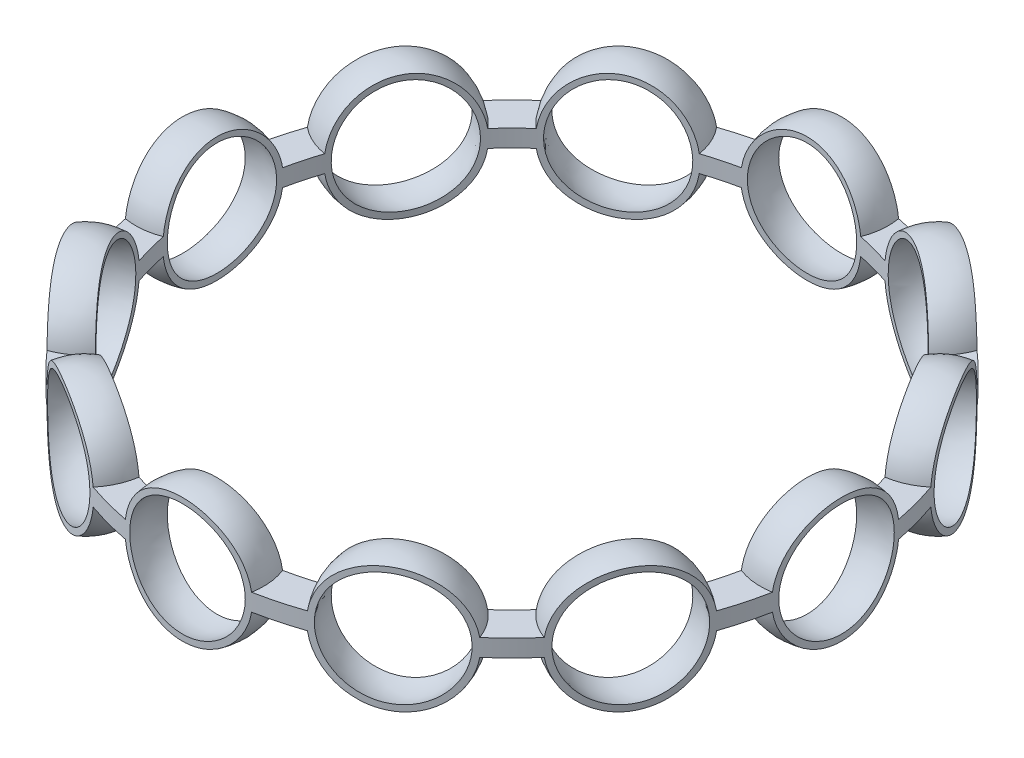
from build123d import *

# Parameters (mm, degrees)
SKETCH1_R               = 50
BOSS_EXTRUDE1_DEPTH     = 1
CIRPATTERN1_COUNT       = 12
CUT_EXTRUDE2_DEPTH      = 72.107313267
CUT_EXTRUDE2_DEPTH_BACK = 72.107313267
SKETCH3_OUTSIDE_W       = 130.442
SKETCH3_OUTSIDE_H       = 130.442
SKETCH3_OUTSIDE_R       = 38.25
SKETCH3_OUTSIDE_R_2     = 34.25
CIRPATTERN2_COUNT       = 12


with BuildPart() as part:
    # Sketch1 → Boss-Extrude1 (new, symmetric)
    with BuildSketch(Plane(origin=(0, 0, 0), x_dir=(1, 0, 0), z_dir=(0, 1, 0))):
        with Locations(Location((0, 0, 0), (0, 0, 270))):
            Circle(SKETCH1_R)
    extrude(amount=BOSS_EXTRUDE1_DEPTH, both=True)

    # Sketch2 → Revolve1 (revolve)
    with BuildSketch(Plane(origin=(0, 0, 0), x_dir=(0, 0, -1), z_dir=(1, 0, 0))):
        with BuildLine():
            Line((36.25, 7.5), (36.25, -7.5))
            ThreePointArc((36.25, -7.5), (43.75, 0), (36.25, 7.5))
        make_face()
    revolve1 = revolve(axis=Axis((0, 22.32089878, -36.25), (0, -1, 0)))

    # CirPattern1: Revolve1 ×12 about axis
    cirpattern1_axis = Axis((0, 0, 0), (0, 1, 0))
    for i in range(1, CIRPATTERN1_COUNT):
        add(revolve1.rotate(cirpattern1_axis, i * 360 / CIRPATTERN1_COUNT))

    # Sketch3 outside → Cut-Extrude2 (cut, two sides: drawn at the far end of the back side and taken through both)
    # profile 1 of 2: a face of its own
    with BuildSketch(Plane(origin=(0, 0, 0), x_dir=(1, 0, 0), z_dir=(0, 1, 0)).offset(-CUT_EXTRUDE2_DEPTH_BACK)):
        Rectangle(SKETCH3_OUTSIDE_W, SKETCH3_OUTSIDE_H)
        with Locations(Location((0, 0, 0), (0, 0, 281.032424599))):
            Circle(SKETCH3_OUTSIDE_R, mode=Mode.SUBTRACT)
    # profile 2 of 2: a face of its own
    with BuildSketch(Plane(origin=(0, 0, 0), x_dir=(1, 0, 0), z_dir=(0, 1, 0)).offset(-CUT_EXTRUDE2_DEPTH_BACK)):
        with Locations(Location((0, 0, 0), (0, 0, 281.660980745))):
            Circle(SKETCH3_OUTSIDE_R_2)
    extrude(amount=CUT_EXTRUDE2_DEPTH + CUT_EXTRUDE2_DEPTH_BACK, mode=Mode.SUBTRACT)

    # Sketch4 → Cut-Revolve1 (revolve, cut)
    with BuildSketch(Plane(origin=(0, 0, 0), x_dir=(0, 0, -1), z_dir=(1, 0, 0))):
        with BuildLine():
            Line((36.25, 6.895296038), (36.25, -6.804703962))
            ThreePointArc((36.25, -6.804703962), (43.1, 0.045296038), (36.25, 6.895296038))
        make_face()
    cut_revolve1 = revolve(axis=Axis((0, 18.089427009, -36.25), (0, -1, 0)), mode=Mode.SUBTRACT)

    # CirPattern2: Cut-Revolve1 ×12 about axis
    cirpattern2_axis = Axis((0, 0, 0), (0, 1, 0))
    for i in range(1, CIRPATTERN2_COUNT):
        add(cut_revolve1.rotate(cirpattern2_axis, i * 360 / CIRPATTERN2_COUNT), mode=Mode.SUBTRACT)


solid = part.part
